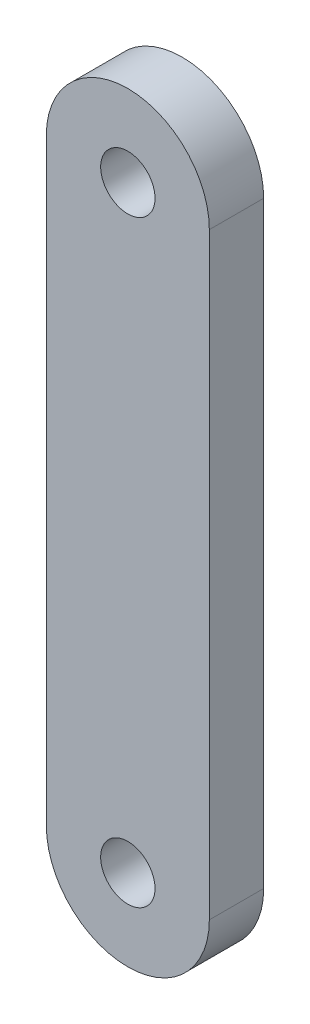
from build123d import *

# Parameters (mm, degrees)
SKETCH_1_R      = 5
EXTRUDE_1_DEPTH = 10


with BuildPart() as part:
    # 草图1 → 凸台-拉伸1 (new body)
    with BuildSketch(Plane.XY):
        with BuildLine():
            Line((-15, 0), (-15, 110))
            ThreePointArc((-15, 110), (0, 125), (15, 110))
            Line((15, 110), (15, 0))
            ThreePointArc((15, 0), (0, -15), (-15, 0))
        make_face()
        Circle(SKETCH_1_R, mode=Mode.SUBTRACT)
        with Locations((0, 110)):
            Circle(SKETCH_1_R, mode=Mode.SUBTRACT)
    extrude(amount=EXTRUDE_1_DEPTH)


solid = part.part
